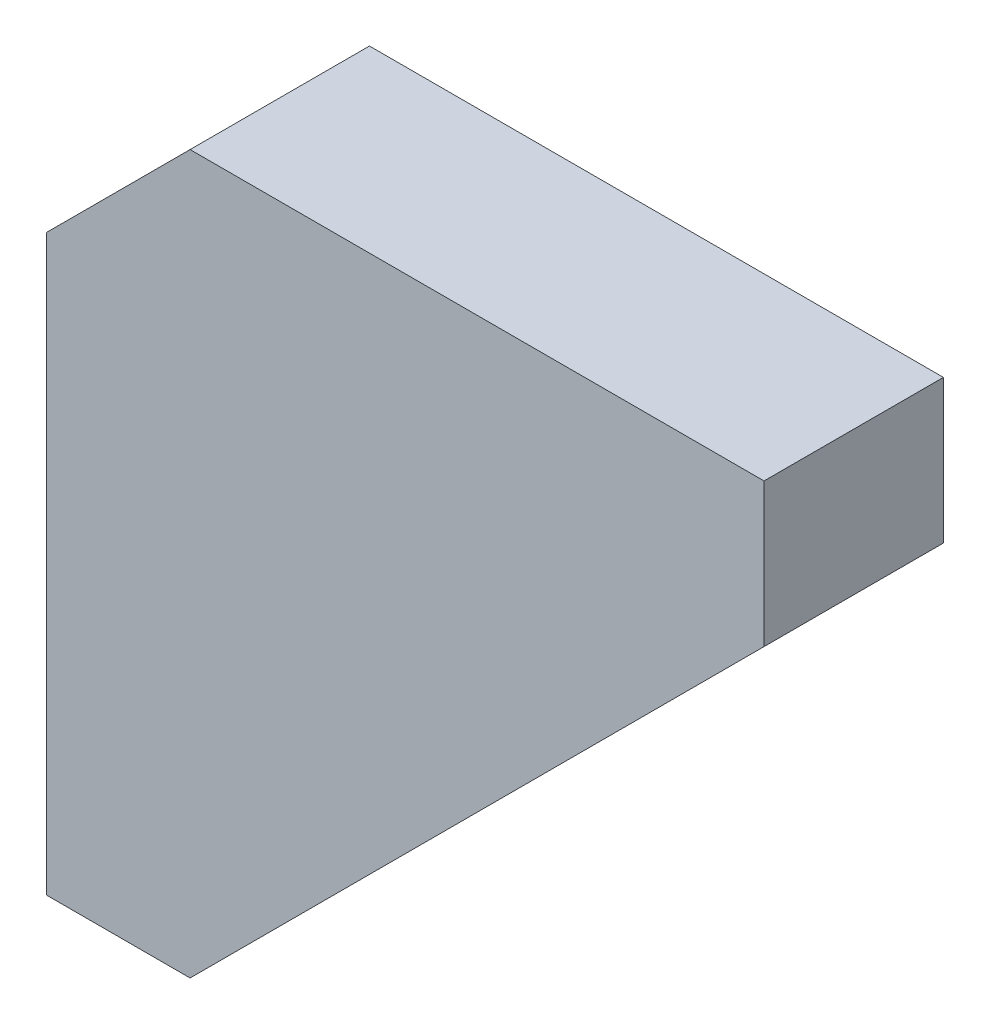
from build123d import *

# Parameters (mm, degrees)
BOSS_EXTRUDE1_DEPTH = 25


with BuildPart() as part:
    # Sketch1 → Boss-Extrude1 (new body)
    with BuildSketch(Plane.XY):
        Polygon((0, 0), (20, 0), (100, 80), (100, 100), (20, 100), (0, 80), align=None)
    extrude(amount=BOSS_EXTRUDE1_DEPTH)


solid = part.part
